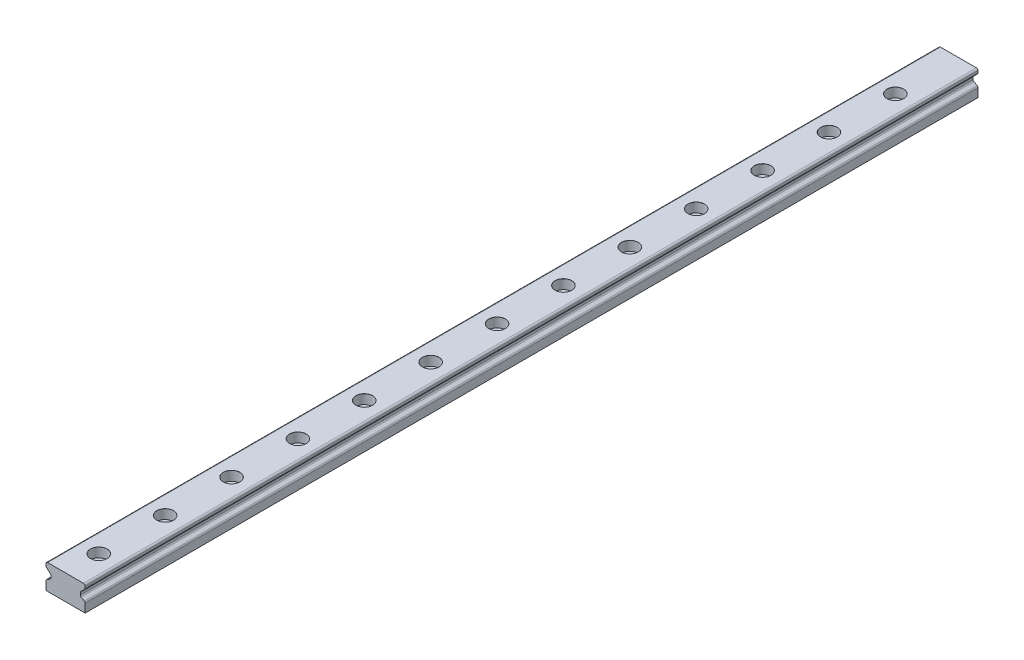
SolidWorks part; units mm, degrees
ref_plane "Front Plane" through (0, 0, 0) normal (0, 0, 1) x (1, 0, 0)
ref_plane "Top Plane" through (0, 0, 0) normal (0, 1, 0) x (1, 0, 0)
ref_plane "Right Plane" through (0, 0, 0) normal (1, 0, 0) x (0, 0, -1)
sketch "Sketch1" plane through (0, 0, 0) normal (0, 0, 1) x (1, 0, 0)
  line L0 (-49.0491, -215.1517) -> (-49.0491, -204.4952) construction
  line L1 (-49.0491, -219.5731) -> (-49.0491, -215.1517) construction
  line L2 (-49.0491, -215.1517) -> (-49.0491, -204.4952)
  line L3 (-49.0491, -219.5731) -> (-49.0491, -215.1517)
  line L12 (-38.2507, -204.4952) -> (-59.8475, -204.4952)
  line L13 (-60.8475, -205.4952) -> (-60.8475, -206.6465)
  line L14 (-60.5298, -207.3776) -> (-58.2267, -209.5269)
  line L15 (-57.909, -210.258) -> (-57.909, -211.561)
  line L16 (-58.4108, -212.428) -> (-60.3457, -213.5398)
  line L17 (-60.8475, -214.4068) -> (-60.8475, -219.5731)
  line L18 (-60.8475, -219.5731) -> (-37.2507, -219.5731)
  line L19 (-37.2507, -219.5731) -> (-37.2507, -214.4068)
  line L20 (-37.7525, -213.5398) -> (-39.6874, -212.428)
  line L21 (-40.1892, -211.561) -> (-40.1892, -210.258)
  line L22 (-39.8715, -209.5269) -> (-37.5684, -207.3776)
  line L23 (-37.2507, -206.6465) -> (-37.2507, -205.4952)
  line L24 (-38.2507, -204.4952) -> (-59.8475, -204.4952)
  line L25 (-60.8475, -205.4952) -> (-60.8475, -206.6465)
  line L26 (-60.5298, -207.3776) -> (-58.2267, -209.5269)
  line L27 (-57.909, -210.258) -> (-57.909, -211.561)
  line L28 (-58.4108, -212.428) -> (-60.3457, -213.5398)
  line L29 (-60.8475, -214.4068) -> (-60.8475, -219.5731)
  line L30 (-60.8475, -219.5731) -> (-37.2507, -219.5731)
  line L31 (-37.2507, -219.5731) -> (-37.2507, -214.4068)
  line L32 (-37.7525, -213.5398) -> (-39.6874, -212.428)
  line L33 (-40.1892, -211.561) -> (-40.1892, -210.258)
  line L34 (-39.8715, -209.5269) -> (-37.5684, -207.3776)
  line L35 (-37.2507, -206.6465) -> (-37.2507, -205.4952)
  arc A10 (-59.8475, -204.4952) -> (-60.8475, -205.4952) centre (-59.8475, -205.4952) ccw
  arc A11 (-60.8475, -206.6465) -> (-60.5298, -207.3776) centre (-59.8475, -206.6465) ccw
  arc A12 (-57.909, -210.258) -> (-58.2267, -209.5269) centre (-58.909, -210.258) ccw
  arc A13 (-58.4108, -212.428) -> (-57.909, -211.561) centre (-58.909, -211.561) ccw
  arc A14 (-60.3457, -213.5398) -> (-60.8475, -214.4068) centre (-59.8475, -214.4068) ccw
  arc A15 (-37.2507, -214.4068) -> (-37.7525, -213.5398) centre (-38.2507, -214.4068) ccw
  arc A16 (-40.1892, -211.561) -> (-39.6874, -212.428) centre (-39.1892, -211.561) ccw
  arc A17 (-39.8715, -209.5269) -> (-40.1892, -210.258) centre (-39.1892, -210.258) ccw
  arc A18 (-37.5684, -207.3776) -> (-37.2507, -206.6465) centre (-38.2507, -206.6465) ccw
  arc A19 (-37.2507, -205.4952) -> (-38.2507, -204.4952) centre (-38.2507, -205.4952) ccw
  arc A20 (-59.8475, -204.4952) -> (-60.8475, -205.4952) centre (-59.8475, -205.4952) ccw
  arc A21 (-60.8475, -206.6465) -> (-60.5298, -207.3776) centre (-59.8475, -206.6465) ccw
  arc A22 (-57.909, -210.258) -> (-58.2267, -209.5269) centre (-58.909, -210.258) ccw
  arc A23 (-58.4108, -212.428) -> (-57.909, -211.561) centre (-58.909, -211.561) ccw
  arc A24 (-60.3457, -213.5398) -> (-60.8475, -214.4068) centre (-59.8475, -214.4068) ccw
  arc A25 (-37.2507, -214.4068) -> (-37.7525, -213.5398) centre (-38.2507, -214.4068) ccw
  arc A26 (-40.1892, -211.561) -> (-39.6874, -212.428) centre (-39.1892, -211.561) ccw
  arc A27 (-39.8715, -209.5269) -> (-40.1892, -210.258) centre (-39.1892, -210.258) ccw
  arc A28 (-37.5684, -207.3776) -> (-37.2507, -206.6465) centre (-38.2507, -206.6465) ccw
  arc A29 (-37.2507, -205.4952) -> (-38.2507, -204.4952) centre (-38.2507, -205.4952) ccw
  dimension "D1" = 0
extrude "Boss-Extrude1" add sketch "Sketch1" along normal blind 538 contours L28 A24 L29 L30 L3 L2 L24 A20 L25 A21 L26 A22 L27 A23 | L35 A29 L24 L2 L3 L30 L31 A25 L32 A26 L33 A27 L34 A28
hole_wizard "CBORE for M5 Hexagon socket head cap screws1" positions "Sketch2" profile "Sketch3" counterbore size "M5" standard "GB" end condition through all
sketch "Sketch2" plane through (0, -204.4952, 0) normal (0, 1, 0) x (1, 0, 0)
  line L0 (-38.2507, -538) -> (-59.8475, -538) construction
  line L1 (-49.0491, -538) -> (-49.0491, -518) construction
  point P0 (-49.0491, -518)
  point P16 (-49.0491, -478)
  point P17 (-49.0491, -438)
  point P18 (-49.0491, -398)
  point P19 (-49.0491, -358)
  point P20 (-49.0491, -318)
  point P21 (-49.0491, -278)
  point P22 (-49.0491, -238)
  point P23 (-49.0491, -198)
  point P24 (-49.0491, -158)
  point P25 (-49.0491, -118)
  point P26 (-49.0491, -78)
  point P27 (-49.0491, -38)
  dimension "D1" = 20
  dimension "D2" = 13
sketch "Sketch3" plane through (-49.0491, -204.4952, 518) normal (1, 0, 0) x (0, 0, 1)
  line L0 (0, 0) -> (0, 15.0778)
  line L1 (0, 15.0778) -> (2.75, 15.0778)
  line L3 (2.75, 15.0778) -> (2.75, 5.7)
  line L4 (5, 5.7) -> (2.75, 5.7)
  line L5 (5, 5.7) -> (5, 0.025)
  line L6 (5, 0.025) -> (5.025, 0)
  line L7 (5.025, 0) -> (0, 0)
  line L8 (-5, 0.025) -> (-5.025, 0) construction
  line L11 (0, -6.35) -> (0, 107.95) construction
  dimension "通孔孔直径" = 5.5
  dimension "通孔孔深度" = 15.0778
  dimension "柱形沉头孔直径" = 10
  dimension "柱形沉头孔深度" = 5.7
  dimension "近端锥形沉头孔直径" = 10.05
  dimension "近端锥形沉头孔角度" = 90
